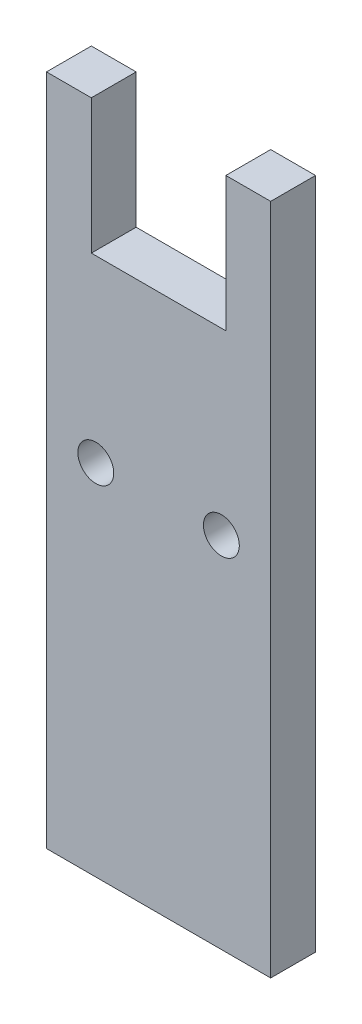
from build123d import *

# Parameters (mm, degrees)
SKETCH1_W           = 50
SKETCH1_H           = 150
BOSS_EXTRUDE1_DEPTH = 10
SKETCH2_W           = 30
SKETCH2_H           = 30
CUT_EXTRUDE1_DEPTH  = 10
SKETCH3_R           = 4
CUT_EXTRUDE2_DEPTH  = 80.686887253


with BuildPart() as part:
    # Sketch1 → Boss-Extrude1 (new body)
    with BuildSketch(Plane.XY):
        Rectangle(SKETCH1_W, SKETCH1_H)
    extrude(amount=BOSS_EXTRUDE1_DEPTH)

    # Sketch2 → Cut-Extrude1 (cut)
    with BuildSketch(Plane.XY.offset(10)):
        with Locations((0, 60)):
            Rectangle(SKETCH2_W, SKETCH2_H)
    extrude(amount=-CUT_EXTRUDE1_DEPTH, mode=Mode.SUBTRACT)

    # Sketch3 → Cut-Extrude2 (cut, through all)
    with BuildSketch(Plane.XY.offset(10)):
        with Locations((-14, 5)):
            Circle(SKETCH3_R)
        with Locations(Location((14, 5, 0), (0, 0, 180))):
            Circle(SKETCH3_R)
    extrude(amount=-CUT_EXTRUDE2_DEPTH, mode=Mode.SUBTRACT)


solid = part.part
